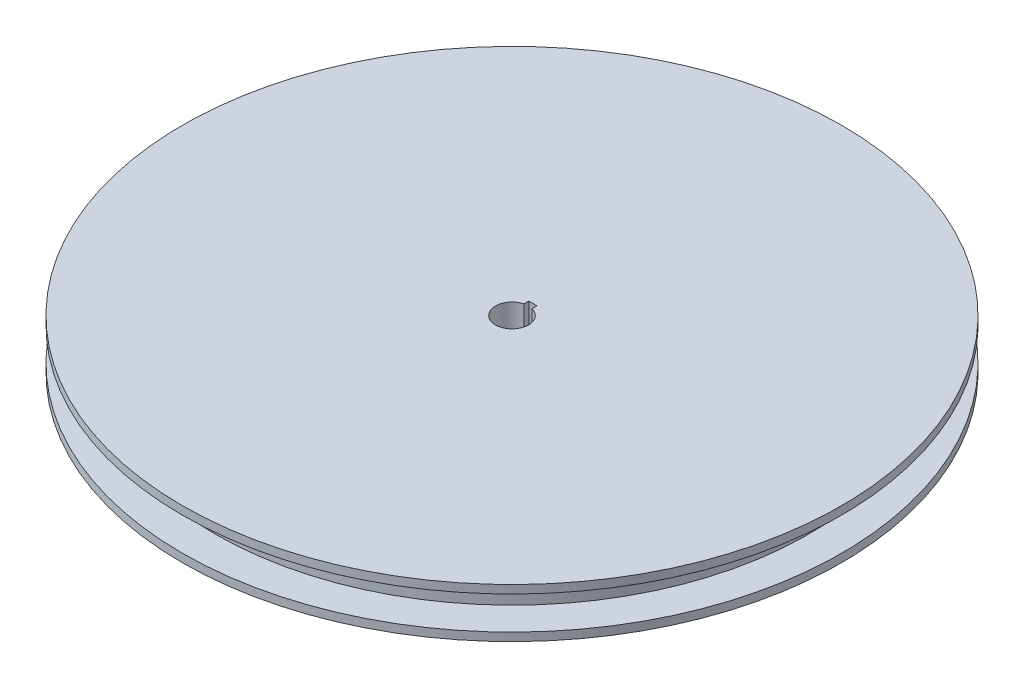
from build123d import *

# Parameters (mm, degrees)
CUT_EXTRUDE1_DEPTH = 285.429253067


with BuildPart() as part:
    # Sketch1 → Revolve1 (revolve)
    with BuildSketch(Plane.XY, mode=Mode.PRIVATE) as revolve1_sk:
        Polygon((-10, 0), (-10, -30), (-200, -30), (-200, -25), (-180, -25), (-180, -5), (-200, -5), (-200, 0), align=None)
    revolve(revolve1_sk.sketch.rotate(Axis((0, 76.758624558, 0), (0, -1, 0)), 270), axis=Axis((0, 76.758624558, 0), (0, -1, 0)))

    # Sketch2 → Cut-Extrude1 (cut, through all)
    with BuildSketch(Plane(origin=(0, 0, 0), x_dir=(1, 0, 0), z_dir=(0, 1, 0))):
        with BuildLine():
            Line((-2.5, 12.682458366), (-2.5, 9.682458366))
            ThreePointArc((-2.5, 9.682458366), (0, 10), (2.5, 9.682458366))
            Line((2.5, 9.682458366), (2.5, 12.682458366))
            Line((2.5, 12.682458366), (-2.5, 12.682458366))
        make_face()
    extrude(amount=-CUT_EXTRUDE1_DEPTH, mode=Mode.SUBTRACT)


solid = part.part
